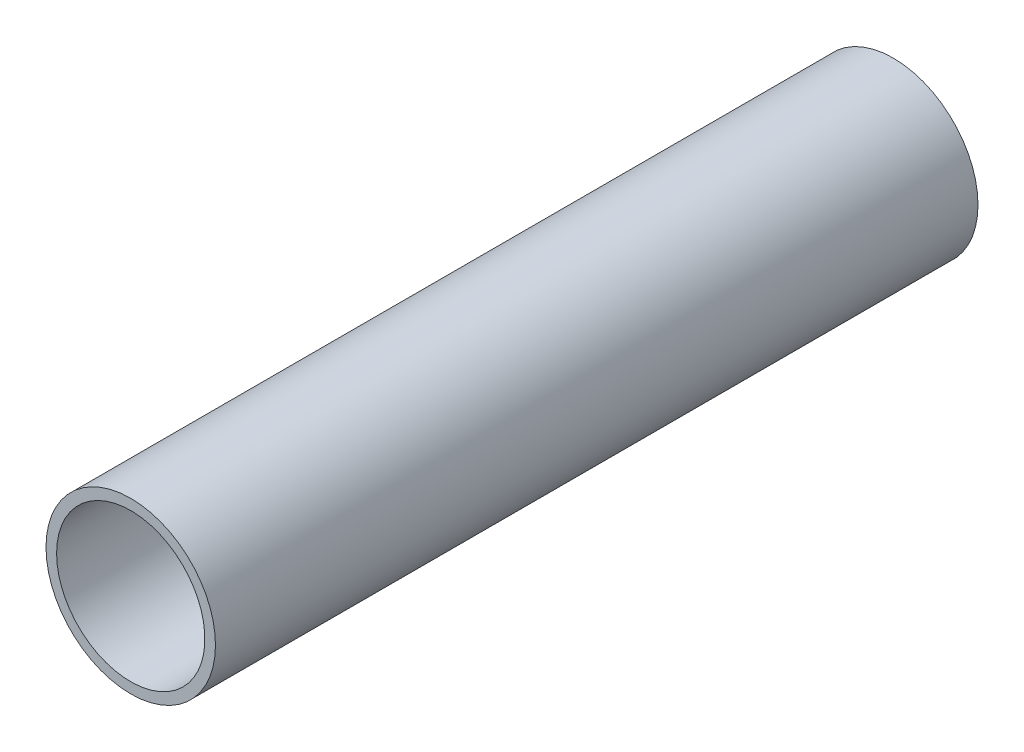
SolidWorks part; units mm, degrees
ref_plane "前视基准面" through (0, 0, 0) normal (0, 0, 1) x (1, 0, 0)
ref_plane "上视基准面" through (0, 0, 0) normal (0, 1, 0) x (1, 0, 0)
ref_plane "右视基准面" through (0, 0, 0) normal (1, 0, 0) x (0, 0, -1)
other "Configuration Table"
sketch "草图1" plane through (0, 0, 0) normal (0, 0, 1) x (1, 0, 0)
  circle A0 centre (0, 0) radius 40
  circle A1 centre (0, 0) radius 35
  dimension "D1" = 70
  dimension "D2" = 80
extrude "凸台-拉伸1" add sketch "草图1" along normal blind 360
